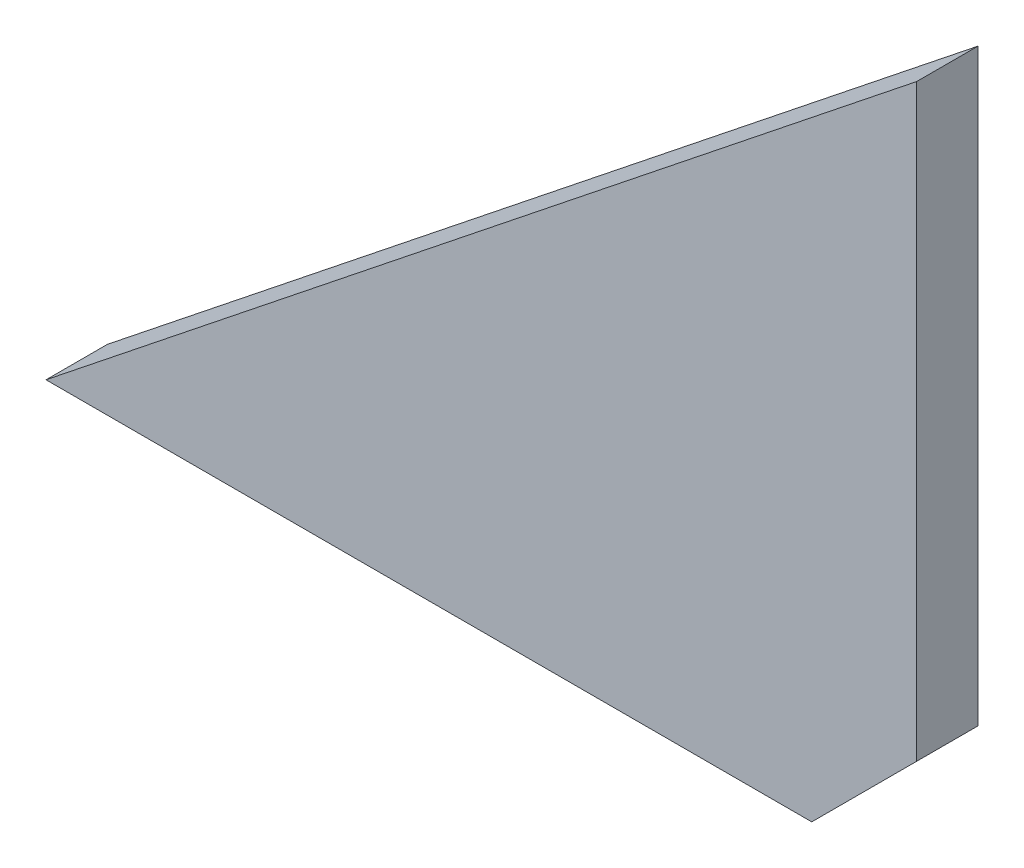
from build123d import *

# Parameters (mm, degrees)
EXTRUDE_1_DEPTH     = 5
SKETCH_2_W          = 100
SKETCH_2_H          = 30
CUT_EXTRUDE_1_DEPTH = 360


with BuildPart() as part:
    # 草图1 → 凸台-拉伸1 (new body)
    with BuildSketch(Plane.XY):
        Polygon((-5, 0), (-5, -47.928932188), (-43.535533906, -86.464466094), (-113.535533906, -86.464466094), align=None)
    extrude(amount=EXTRUDE_1_DEPTH)

    # 草图2 → 切除-拉伸1 (cut)
    with BuildSketch(Plane.XY.offset(5)):
        with Locations((-63.535533906, -71.464466094)):
            Rectangle(SKETCH_2_W, SKETCH_2_H)
    extrude(amount=-CUT_EXTRUDE_1_DEPTH, mode=Mode.SUBTRACT)


solid = part.part
